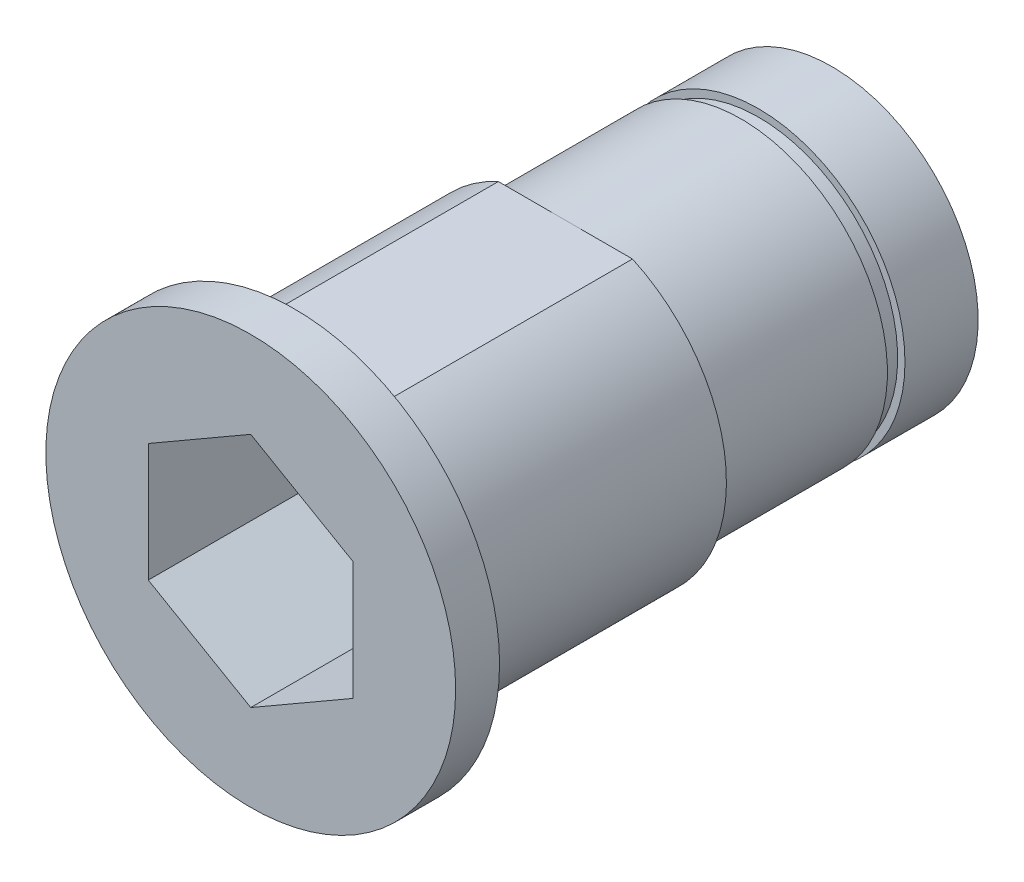
SolidWorks part; units mm, degrees
ref_plane "前视基准面" through (0, 0, 0) normal (0, 0, 1) x (1, 0, 0)
ref_plane "上视基准面" through (0, 0, 0) normal (0, 1, 0) x (1, 0, 0)
ref_plane "右视基准面" through (0, 0, 0) normal (1, 0, 0) x (0, 0, -1)
sketch "草图1" plane through (0, 0, 0) normal (0, 0, 1) x (1, 0, 0)
  circle A0 centre (0, 0) radius 6
  circle A1 centre (0, 0) radius 11
  dimension "D1" = 12
  dimension "D2" = 22
extrude "凸台-拉伸1" add sketch "草图1" along normal blind 34
sketch "草图2" plane through (0, 0, 34) normal (0, 0, 1) x (1, 0, 0)
  circle A0 centre (0, 0) radius 7
  circle A1 centre (0, 0) radius 14
  dimension "D1" = 28
  dimension "D2" = 14
extrude "凸台-拉伸2" add sketch "草图2" along normal blind 3
sketch "草图3" plane through (0, 0, 0) normal (0, 0, -1) x (-1, 0, 0)
  circle A0 centre (0, 0) radius 12.0173
  circle A1 centre (0, 0) radius 10
  dimension "D1" = 20
extrude "切除-拉伸1" cut sketch "草图3" against normal blind 15.5
sketch "草图4" plane through (0, 0, 0) normal (0, 0, -1) x (-1, 0, 0)
  line L0 (-5.4204, 10) -> (-5.4204, 11.9776)
  line L1 (-5.4204, 11.9776) -> (7.8159, 11.9776)
  line L2 (7.8159, 11.9776) -> (7.8159, 10)
  line L3 (7.8159, 10) -> (-5.4204, 10)
extrude "切除-拉伸2" cut sketch "草图4" against normal blind 32
sketch "草图5" plane through (0, 0, 37) normal (0, 0, 1) x (1, 0, 0)
  line L0 (0, 2.6108) -> (0, -11.752) construction
  line L1 (7, -4.0415) -> (7, 4.0415)
  line L2 (7, 4.0415) -> (0, 8.0829)
  line L3 (0, 8.0829) -> (-7, 4.0415)
  line L4 (-7, 4.0415) -> (-7, -4.0415)
  line L5 (-7, -4.0415) -> (0, -8.0829)
  line L6 (0, -8.0829) -> (7, -4.0415)
  circle A1 centre (0, 0) radius 7 construction
  dimension "D1" = 14
extrude "切除-拉伸3" cut sketch "草图5" against normal through all
sketch "草图6" plane through (0, 0, 0) normal (0, 1, 0) x (1, 0, 0)
  line L0 (10, -15.5) -> (10, 0) construction
  line L1 (9.5, -2.3) -> (10.5, -2.3)
  line L2 (9.5, -2.3) -> (9.5, -3.5)
  line L3 (9.5, -3.5) -> (10.5, -3.5)
  line L4 (10.5, -2.3) -> (10.5, -3.5)
  line L5 (9.5, -2.3) -> (10.5, -3.5) construction
  line L6 (9.5, -3.5) -> (10.5, -2.3) construction
  line L7 (10, 0) -> (-10, 0) construction
  line L8 (0, 1.6951) -> (0, -1.2117) construction
  point P0 (10, -2.9)
  dimension "D1" = 3.5
  dimension "D2" = 1.2
  dimension "D3" = 1
revolve "切除-旋转1" cut sketch "草图6" angle 360 about L8
sketch "草图7" plane through (0, 0, 0) normal (0, 0, -1) x (-1, 0, 0)
  line L0 (0, -8.0829) -> (-7, -4.0415) construction
  line L1 (7, -4.0415) -> (7, 4.0415)
  line L2 (7, 4.0415) -> (0, 8.0829)
  line L3 (0, 8.0829) -> (-7, 4.0415)
  line L4 (-7, 4.0415) -> (-7, -4.0415)
  line L5 (-7, -4.0415) -> (0, -8.0829)
  line L6 (0, -8.0829) -> (7, -4.0415)
  circle A0 centre (0, 0) radius 10
  circle A1 centre (0, 0) radius 7 construction
  circle A2 centre (0, 0) radius 10 construction
extrude "凸台-拉伸3" add sketch "草图7" along normal blind 2.7
